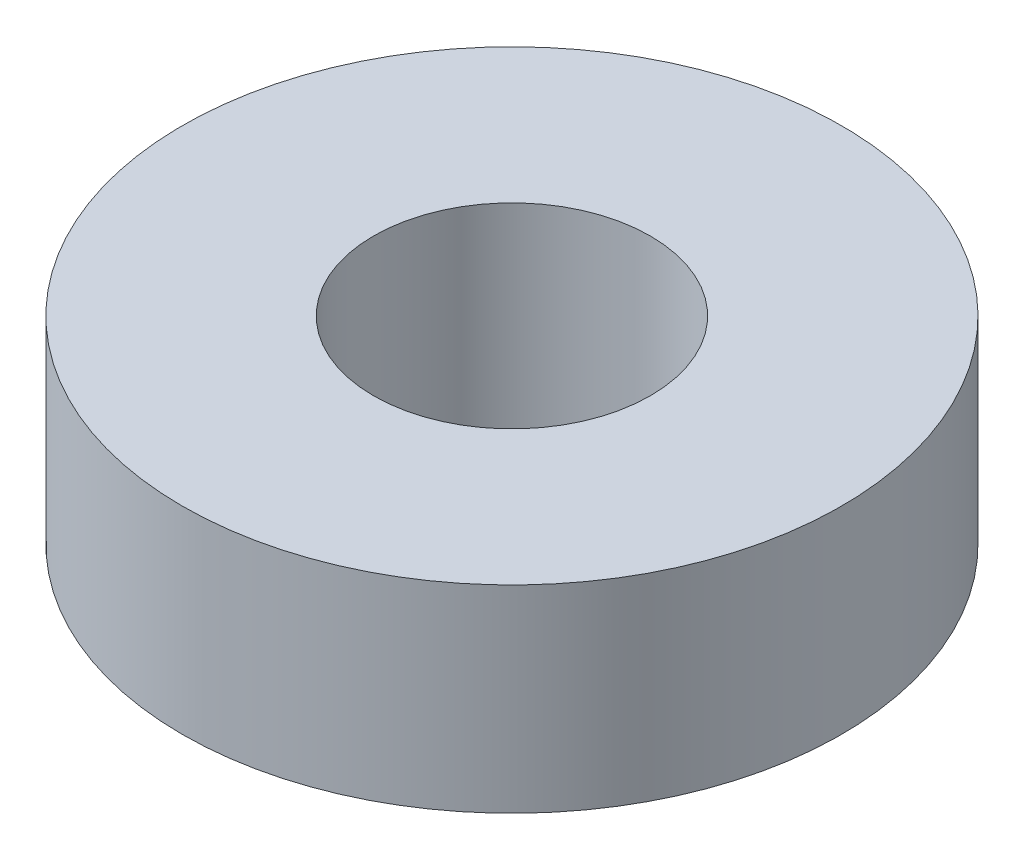
SolidWorks part; units mm, degrees
ref_plane "前视基准面" through (0, 0, 0) normal (0, 0, 1) x (1, 0, 0)
ref_plane "上视基准面" through (0, 0, 0) normal (0, 1, 0) x (1, 0, 0)
ref_plane "右视基准面" through (0, 0, 0) normal (1, 0, 0) x (0, 0, -1)
other "Configuration Table"
sketch "草图1" plane through (0, 0, 0) normal (0, 1, 0) x (1, 0, 0)
  circle A0 centre (0, 0) radius 5
  circle A1 centre (0, 0) radius 2.1
  dimension "D1" = 10
  dimension "D2" = 4.2
extrude "凸台-拉伸1" add sketch "草图1" along normal blind 3
